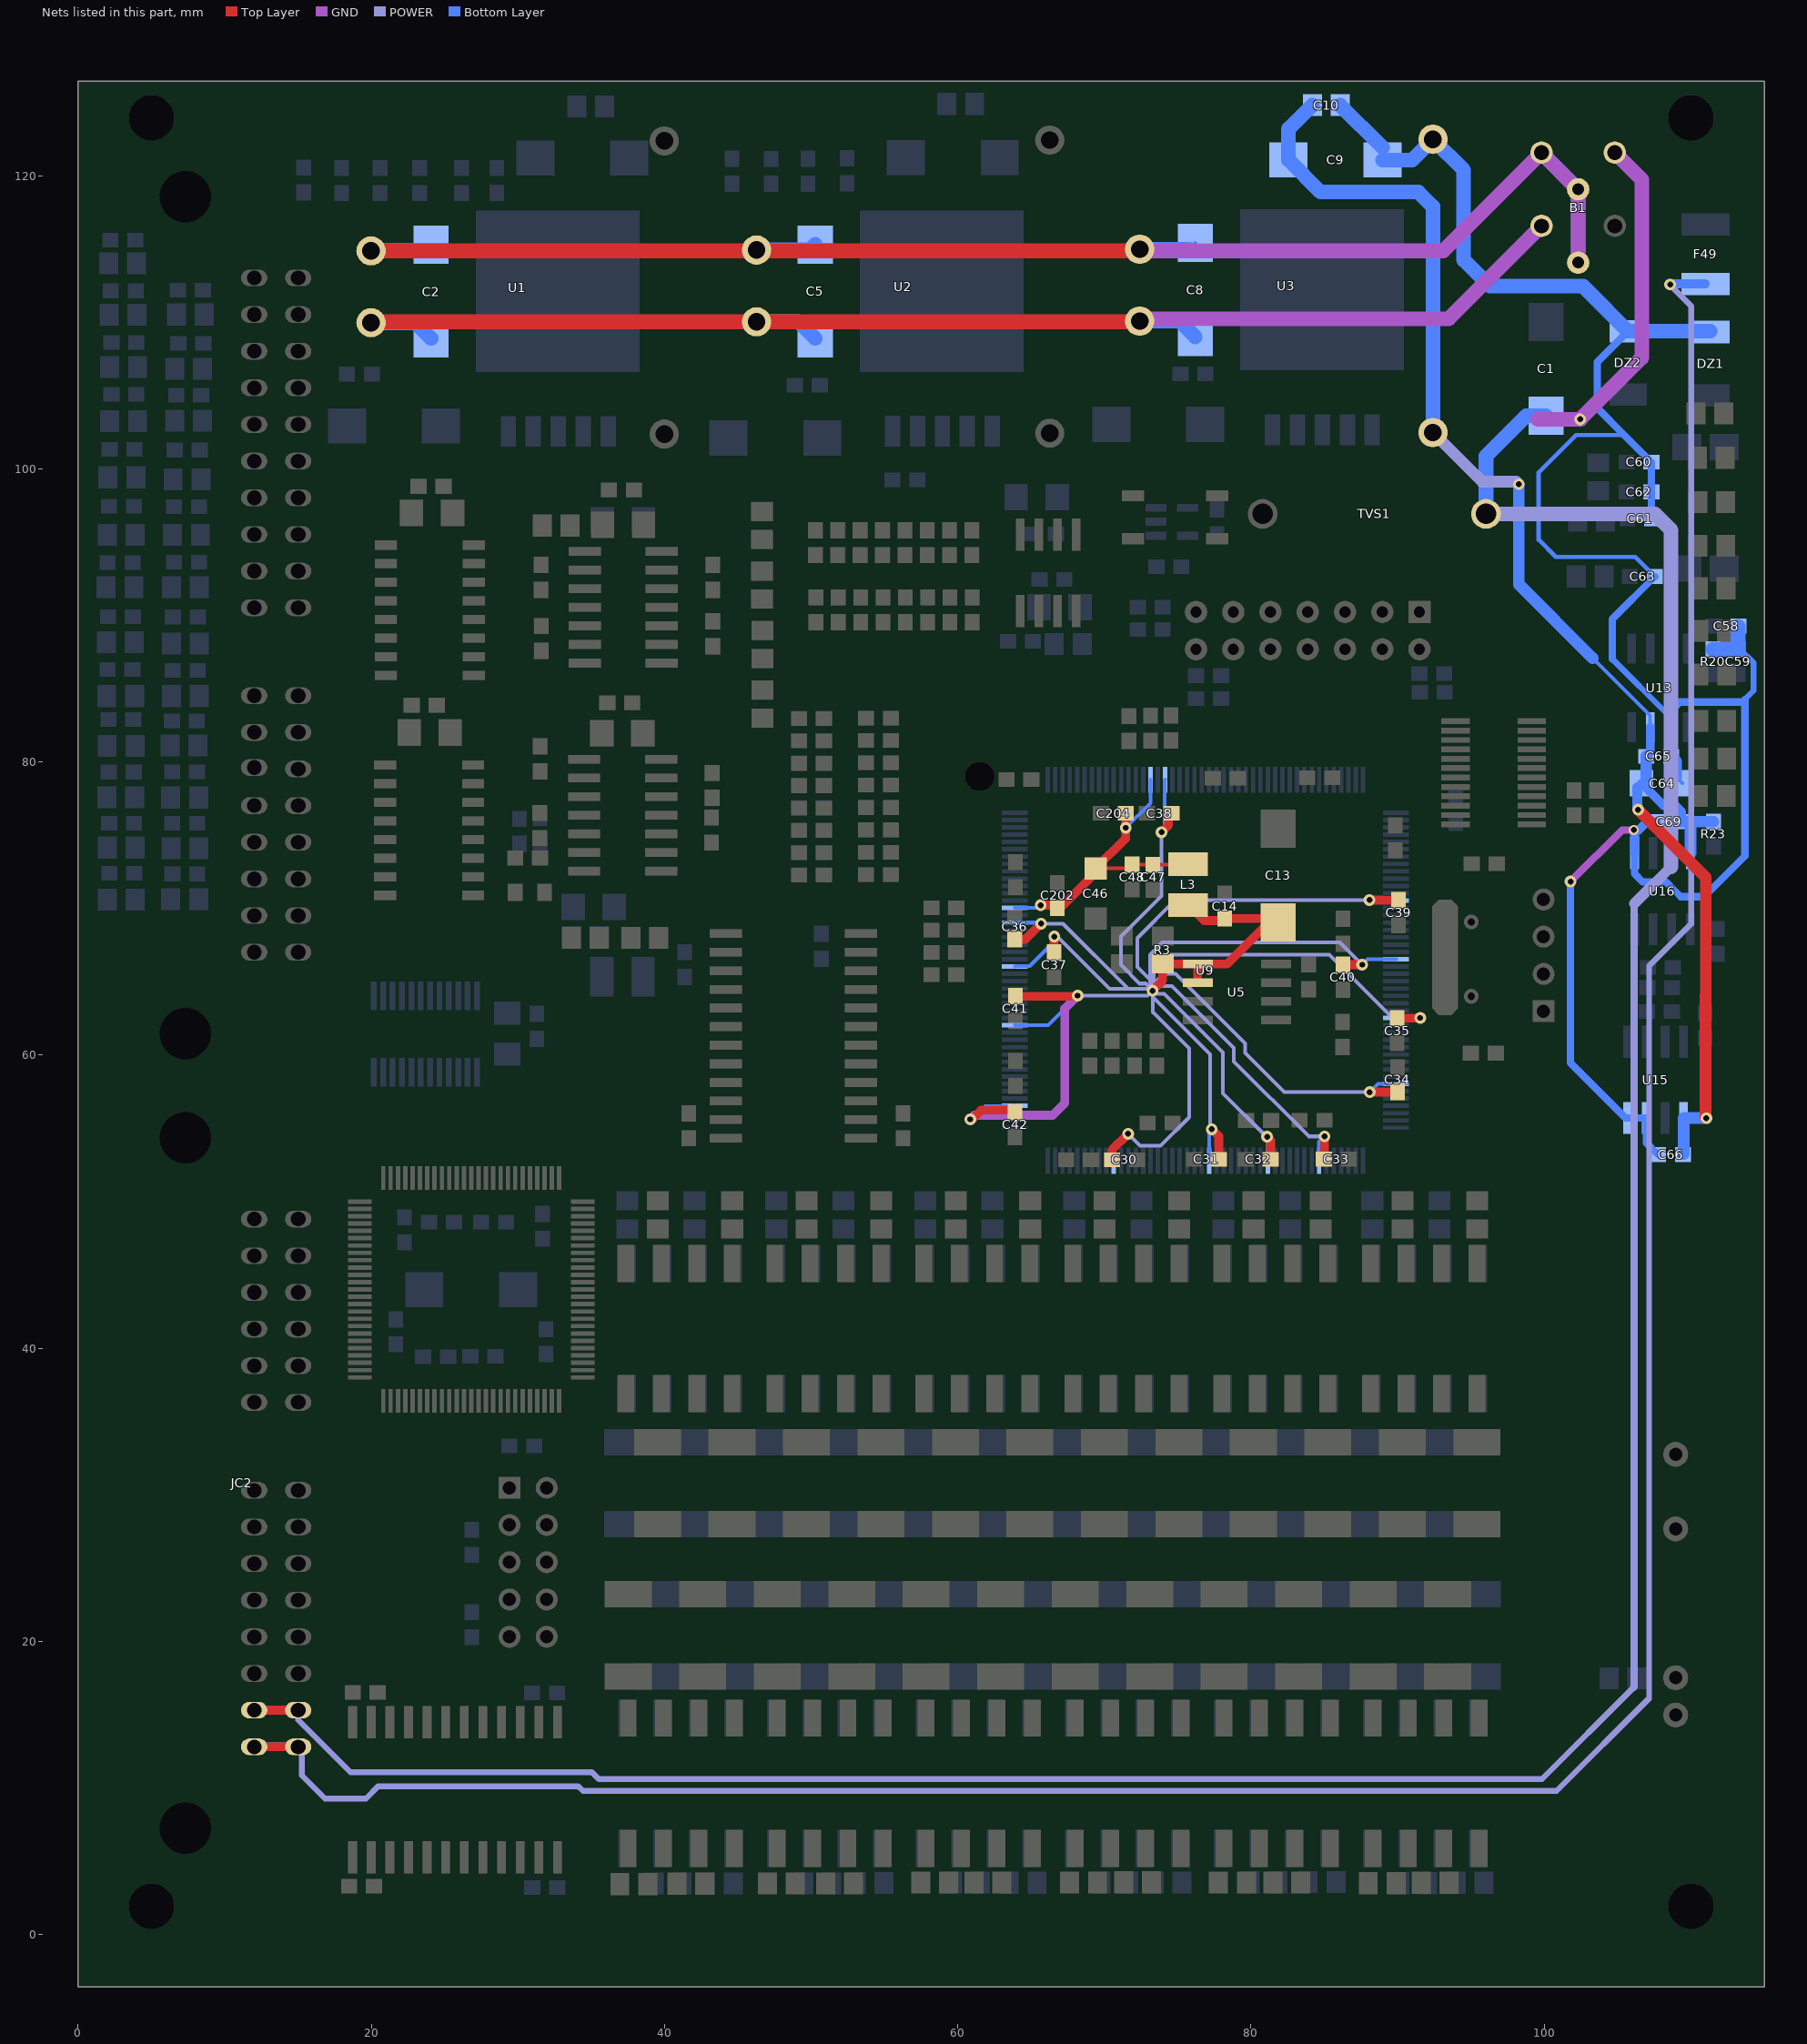
[diagram p0: the nets of this part, all layers, seen from the top]
# Altium PCB MISC86180.PCBDOC (part 3 of 9)
Units mm, origin at the board's own origin, x right, y up, seen from the top; angles counter-clockwise.
Board outline 115 x 130 mm, 4 copper layers (Top Layer, GND, POWER, Bottom Layer); 475 components, 355 nets, 1755 pads, 459 vias.

## Footprints (in the part's own frame and the unit in brackets; to place one, negate y for a bottom-side part, rotate by r counter-clockwise, add the part's x,y. Pads: shape width x height; smd on the part's side, far side on the other; paste and mask are expansions set on the pad) (continued)
AQZ102 [mm]
  round 1.7 hole 0.9: 1(1.275,-1.026) 2(3.815,-1.026) 3(13.975,-1.026) 4(19.055,-1.026)
  silkscreen extent 0,-3.06 20.32,-0.01
BNX012H [mm]
  round 1.524 hole 1: 1(-3,-3) 2(-3,-8) 3(-8,-3) 4(-8,-8)
  round 1.524 hole 0.8: 5(-5.5,-5.5) 6(-0.5,-5.5)
  silkscreen extent -12.19,-11.05 0,0
CR1608-0603 [mm]
  rect 1.1x1 smd: 1(-0.85,-0.018) 2(0.85,-0.018)
CR2012-0805 [mm]
  rect 1.3x1.5 smd: 1(-0.941,-0.018) 2(0.959,-0.018)
CR3216-1206 [mm]
  rect 1.6x1.8 smd: 1(-1.391,-0.018) 2(1.409,-0.018)
  silkscreen extent -0.29,-0.82 0.31,0.78
CR3225-1210 [mm]
  rect 1.6x2.7 smd: 1(-1.395,0.005) 2(1.405,0.005)
  silkscreen extent -0.3,-1.25 0.3,1.25
CR6332-2512 [mm] "Chip Resistor; Body 6.3 x 3.2 mm (LxW typ)"
  rect 1.8x3.2 smd: 1(-2.8,0) 2(2.8,0)
  silkscreen extent -1.6,-1.5 1.6,1.5
D008 [mm]
  rect 0.6x2.05 smd: 1(-1.9,-2.673) 2(-0.63,-2.673) 3(0.64,-2.673) 4(1.91,-2.673) 5(1.91,2.677) 6(0.64,2.677) 7(-0.63,2.677) 8(-1.9,2.677)
  silkscreen extent -2.88,-2.8 2.5,1.25
DBQ024 [mm]
  rect 0.4x1.95 smd: 1(-3.522,-2.616) 2(-2.882,-2.616) 3(-2.242,-2.616) 4(-1.602,-2.616) 5(-0.962,-2.616) 6(-0.322,-2.616) 7(0.318,-2.616) 8(0.958,-2.616) 9(1.598,-2.616) 10(2.238,-2.616) 11(2.878,-2.616) 12(3.518,-2.616) 13(3.518,2.584) 14(2.878,2.584) 15(2.238,2.584) 16(1.598,2.584) 17(0.958,2.584) 18(0.318,2.584) 19(-0.322,2.584) 20(-0.962,2.584) 21(-1.602,2.584) 22(-2.242,2.584) 23(-2.882,2.584) 24(-3.522,2.584)
  silkscreen extent -4.4,-2.74 4.37,1.21
DBV005 [mm]
  rect 0.55x1.45 smd: 1(-0.941,-1.094) 2(0.009,-1.094) 3(0.959,-1.094) 4(0.959,1.056) 5(-0.941,1.056)
  silkscreen extent -1.57,-1.37 1.56,0.88
DCDC_5W [mm]
  round 2 hole 1.2: 1(14.991,-15.832) 2(14.991,-10.932) 3(34.991,-23.432) 4(34.991,-3.432)
  silkscreen extent 12.05,-26.01 37.5,-0.01
FUSE [mil]
  rect 60x130 smd: 1(10.18,-65.41) 2(170.18,-65.41)
  silkscreen extent 0,-135 180,5
HDR1X4 [mm] "Connector; Header; 4 Position"
  rect 1.5x1.5 hole 0.9: 1(0,0)
  round 1.5 hole 0.9: 2(2.54,0) 3(5.08,0) 4(7.62,0)
  silkscreen extent -1.27,-1.27 8.89,1.27
HDR2X5 [mm]
  rect 1.5x1.5 hole 0.9: 1(0.005,0.005)
  round 1.5 hole 0.9: 2(0.005,2.545) 3(2.545,0.005) 4(2.545,2.545) 5(5.085,0.005) 6(5.085,2.545) 7(7.625,0.005) 8(7.625,2.545) 9(10.165,0.005) 10(10.165,2.545)
  silkscreen extent -1.27,-1.27 11.43,3.81
INDC2012-0805 [mm]
  rect 1x1.2 smd: 1(-0.995,-0.008) 2(1.005,-0.008)
  silkscreen extent -0.2,-0.51 0.2,0.49
JTAG14 [mil]
  rect 60x60 hole 30: 1(0,0)
  round 60 hole 30: 2(0,100) 3(100,0) 4(100,100) 5(200,0) 6(200,100) 7(300,0) 8(300,100) 9(400,0) 10(400,100) 11(500,0) 12(500,100) 13(600,0) 14(600,100)
  silkscreen extent -200,-125 800,225
Oscillator [mil]
  round 40 hole 20: 1(-200.19,-0.02) 2(-0.19,-0.02)
  oct 310x70 smd: 3(-105.19,-70.02)
  silkscreen extent -310,-85 110,85
QFP176NEW [mm]
  rect 0.3x1.778 smd: 1(-0.003,-0.011) 2(0.497,-0.011) 3(0.997,-0.011) 4(1.497,-0.011) 5(1.997,-0.011) 6(2.497,-0.011) 7(2.997,-0.011) 8(3.497,-0.011) 9(3.997,-0.011) 10(4.497,-0.011) 11(4.997,-0.011) 12(5.497,-0.011) 13(5.997,-0.011) 14(6.497,-0.011) 15(6.997,-0.011) 16(7.497,-0.011) 17(7.997,-0.011) 18(8.497,-0.011) 19(8.997,-0.011) 20(9.497,-0.011) 21(9.997,-0.011) 22(10.497,-0.011) 23(10.997,-0.011) 24(11.497,-0.011) 25(11.997,-0.011) 26(12.497,-0.011) 27(12.997,-0.011) 28(13.497,-0.011) 29(13.997,-0.011) 30(14.497,-0.011) 31(14.997,-0.011) 32(15.497,-0.011) 33(15.997,-0.011) 34(16.497,-0.011) 35(16.997,-0.011) 36(17.497,-0.011) 37(17.997,-0.011) 38(18.497,-0.011) 39(18.997,-0.011) 40(19.497,-0.011) 41(19.997,-0.011) 42(20.497,-0.011) 43(20.997,-0.011) 44(21.497,-0.011) 89(21.497,25.989) 90(20.997,25.989) 91(20.497,25.989) 92(19.997,25.989) 93(19.497,25.989) 94(18.997,25.989) 95(18.497,25.989) 96(17.997,25.989) 97(17.497,25.989) 98(16.997,25.989) 99(16.497,25.989) 100(15.997,25.989) 101(15.497,25.989) 102(14.997,25.989) 103(14.497,25.989) 104(13.997,25.989) 105(13.497,25.989) 106(12.997,25.989) 107(12.497,25.989) 108(11.997,25.989) 109(11.497,25.989) 110(10.997,25.989) 111(10.497,25.989) 112(9.997,25.989) 113(9.497,25.989) 114(8.997,25.989) 115(8.497,25.989) 116(7.997,25.989) 117(7.497,25.989) 118(6.997,25.989) 119(6.497,25.989) 120(5.997,25.989) 121(5.497,25.989) 122(4.997,25.989) 123(4.497,25.989) 124(3.997,25.989) 125(3.497,25.989) 126(2.997,25.989) 127(2.497,25.989) 128(1.997,25.989) 129(1.497,25.989) 130(0.997,25.989) 131(0.497,25.989) 132(-0.003,25.989)
  rect 1.778x0.3 smd: 45(23.747,2.239) 46(23.747,2.739) 47(23.747,3.239) 48(23.747,3.739) 49(23.747,4.239) 50(23.747,4.739) 51(23.747,5.239) 52(23.747,5.739) 53(23.747,6.239) 54(23.747,6.739) 55(23.747,7.239) 56(23.747,7.739) 57(23.747,8.239) 58(23.747,8.739) 59(23.747,9.239) 60(23.747,9.739) 61(23.747,10.239) 62(23.747,10.739) 63(23.747,11.239) 64(23.747,11.739) 65(23.747,12.239) 66(23.747,12.739) 67(23.747,13.239) 68(23.747,13.739) 69(23.747,14.239) 70(23.747,14.739) 71(23.747,15.239) 72(23.747,15.739) 73(23.747,16.239) 74(23.747,16.739) 75(23.747,17.239) 76(23.747,17.739) 77(23.747,18.239) 78(23.747,18.739) 79(23.747,19.239) 80(23.747,19.739) 81(23.747,20.239) 82(23.747,20.739) 83(23.747,21.239) 84(23.747,21.739) 85(23.747,22.239) 86(23.747,22.739) 87(23.747,23.239) 88(23.747,23.739) 133(-2.253,23.739) 134(-2.253,23.239) 135(-2.253,22.739) 136(-2.253,22.239) 137(-2.253,21.739) 138(-2.253,21.239) 139(-2.253,20.739) 140(-2.253,20.239) 141(-2.253,19.739) 142(-2.253,19.239) 143(-2.253,18.739) 144(-2.253,18.239) 145(-2.253,17.739) 146(-2.253,17.239) 147(-2.253,16.739) 148(-2.253,16.239) 149(-2.253,15.739) 150(-2.253,15.239) 151(-2.253,14.739) 152(-2.253,14.239) 153(-2.253,13.739) 154(-2.253,13.239) 155(-2.253,12.739) 156(-2.253,12.239) 157(-2.253,11.739) 158(-2.253,11.239) 159(-2.253,10.739) 160(-2.253,10.239) 161(-2.253,9.739) 162(-2.253,9.239) 163(-2.253,8.739) 164(-2.253,8.239) 165(-2.253,7.739) 166(-2.253,7.239) 167(-2.253,6.739) 168(-2.253,6.239) 169(-2.253,5.739) 170(-2.253,5.239) 171(-2.253,4.739) 172(-2.253,4.239) 173(-2.253,3.739) 174(-2.253,3.239) 175(-2.253,2.739) 176(-2.253,2.239)
  silkscreen extent -2.02,-0.51 22.35,24.88
SB560 [mil]
  round 80 hole 55: 1(0.18,-0.41) 2(600.18,-0.41)
  silkscreen extent 0,-100 600,100
SO16 [mm]
  rect 1.5x0.635 smd: 1(-0.007,-0.002) 2(-0.007,-1.272) 3(-0.007,-2.542) 4(-0.007,-3.812) 5(-0.007,-5.082) 6(-0.007,-6.352) 7(-0.007,-7.622) 8(-0.007,-8.892) 9(5.993,-8.892) 10(5.993,-7.622) 11(5.993,-6.352) 12(5.993,-5.082) 13(5.993,-3.812) 14(5.993,-2.542) 15(5.993,-1.272) 16(5.993,-0.002)
  silkscreen extent 0.99,-9.58 4.99,0.69
SO-G8 [mm]
  rect 0.6x2.2 smd: 1(-1.893,-2.599) 2(-0.623,-2.599) 3(0.647,-2.599) 4(1.917,-2.599) 5(1.917,2.601) 6(0.647,2.601) 7(-0.623,2.601) 8(-1.893,2.601)
  silkscreen extent -2.87,-2.72 2.51,1.1
SW_RESET [mil]
  rect 60x30 smd: 1(-25,-30) 2(-25,-145) 3(201,-145) 4(201,-30)
  silkscreen extent 0,-176 176,0
TC7343-2917 [mm]
  rect 2.6x2.4 smd: 1(-3.194,-0.018) 2(3.206,-0.018)
  silkscreen extent -4.57,-2.32 3.81,2.41
TQFP100 [mm]
  rect 1.6x0.3 smd: 1(-7.6,6) 2(-7.6,5.5) 3(-7.6,5) 4(-7.6,4.5) 5(-7.6,4) 6(-7.6,3.5) 7(-7.6,3) 8(-7.6,2.5) 9(-7.6,2) 10(-7.6,1.5) 11(-7.6,1) 12(-7.6,0.5) 13(-7.6,0) 14(-7.6,-0.5) 15(-7.6,-1) 16(-7.6,-1.5) 17(-7.6,-2) 18(-7.6,-2.5) 19(-7.6,-3) 20(-7.6,-3.5) 21(-7.6,-4) 22(-7.6,-4.5) 23(-7.6,-5) 24(-7.6,-5.5) 25(-7.6,-6) 51(7.6,-6) 52(7.6,-5.5) 53(7.6,-5) 54(7.6,-4.5) 55(7.6,-4) 56(7.6,-3.5) 57(7.6,-3) 58(7.6,-2.5) 59(7.6,-2) 60(7.6,-1.5) 61(7.6,-1) 62(7.6,-0.5) 63(7.6,0) 64(7.6,0.5) 65(7.6,1) 66(7.6,1.5) 67(7.6,2) 68(7.6,2.5) 69(7.6,3) 70(7.6,3.5) 71(7.6,4) 72(7.6,4.5) 73(7.6,5) 74(7.6,5.5) 75(7.6,6)
  rect 0.3x1.6 smd: 26(-6,-7.6) 27(-5.5,-7.6) 28(-5,-7.6) 29(-4.5,-7.6) 30(-4,-7.6) 31(-3.5,-7.6) 32(-3,-7.6) 33(-2.5,-7.6) 34(-2,-7.6) 35(-1.5,-7.6) 36(-1,-7.6) 37(-0.5,-7.6) 38(0,-7.6) 39(0.5,-7.6) 40(1,-7.6) 41(1.5,-7.6) 42(2,-7.6) 43(2.5,-7.6) 44(3,-7.6) 45(3.5,-7.6) 46(4,-7.6) 47(4.5,-7.6) 48(5,-7.6) 49(5.5,-7.6) 50(6,-7.6) 76(6,7.6) 77(5.5,7.6) 78(5,7.6) 79(4.5,7.6) 80(4,7.6) 81(3.5,7.6) 82(3,7.6) 83(2.5,7.6) 84(2,7.6) 85(1.5,7.6) 86(1,7.6) 87(0.5,7.6) 88(0,7.6) 89(-0.5,7.6) 90(-1,7.6) 91(-1.5,7.6) 92(-2,7.6) 93(-2.5,7.6) 94(-3,7.6) 95(-3.5,7.6) 96(-4,7.6) 97(-4.5,7.6) 98(-5,7.6) 99(-5.5,7.6) 100(-6,7.6)
  silkscreen extent -7.72,-6.4 6.4,6.82
WSO24 [mm] "Small Outline; 24 Leads; Body Width 7.5 mm; Pitch 1.27 mm"
  rect 0.6x2.2 smd: 1(-6.985,-4.6) 2(-5.715,-4.6) 3(-4.445,-4.6) 4(-3.175,-4.6) 5(-1.905,-4.6) 6(-0.635,-4.6) 7(0.635,-4.6) 8(1.905,-4.6) 9(3.175,-4.6) 10(4.445,-4.6) 11(5.715,-4.6) 12(6.985,-4.6) 13(6.985,4.6) 14(5.715,4.6) 15(4.445,4.6) 16(3.175,4.6) 17(1.905,4.6) 18(0.635,4.6) 19(-0.635,4.6) 20(-1.905,4.6) 21(-3.175,4.6) 22(-4.445,4.6) 23(-5.715,4.6) 24(-6.985,4.6)
  silkscreen extent -7.96,-4.73 7.93,3.1
ZJYS [mm]
  rect 1.8x2 smd: 1(0.009,-0.015) 2(0.009,-2.555) 3(8.309,-2.555) 4(8.309,-0.015)
  silkscreen extent 1.74,-3.83 6.57,1.25

## Part data
C1 C2 C3 C5 C6 C8 C9 C11 C13 C15 C17 C81: "Polarized Capacitor (Surface Mount)"
C4 C7 C10 C12 C14 C16 C18 C19 C20 C21 C22 C23 C24 C25 C26 C27 C28 C29 C30 C31 C32 C33 C34 C35 C36 C37 C38 C39 C40 C41 C42 C46 C47 C48 C52 C53 C54 C55 C56 C57 C58 C59 C60 C61 C62 C63 C64 C65 C66 C67 C68 C69 C82 C83 C84 C85 C86 C87 C88 C89 C90 C91 C92 C93 C94 C95 C96 C97 C98 C99 C100 C101 C102 C103 C104 C105 C106 C107 C108 C109 C110 C111 C112 C113 C114 C115 C116 C117 C118 C119 C120 C121 C122 C123 C124 C125 C126 C127 C128 C129 C130 C131 C132 C133 C134 C135 C136 C137 C138 C139 C140 C141 C142 C143 C144 C145 C146 C147 C148 C149 C150 C151 C152 C153 C154 C155 C156 C157 C158 C159 C160 C161 C162 C163 C164 C165 C166 C167 C168 C169 C170 C171 C172 C173 C174 C175 C176 C177 C178 C179 C180 C181 C182 C183 C184 C185 C186 C187 C188 C189 C191 C192 C195 C196 C197 C199 C200 C201 C202 C203 C204 C205 C206 C208 C209: "Capacitor"
D1 D2 D3 D4 D5 D6 D7 D8 D9 D10: library part LED1, "Typical YELLOW GaAs LED"
DZ1 DZ2: library part AK1B
F1 F2 F3 F4 F5 F6 F7 F8 F9 F10 F11 F12 F13 F14 F15 F16 F17 F18 F19 F20 F21 F22 F23 F24 F25 F26 F27 F28 F29 F30 F31 F32 F33 F34 F35 F36 F37 F38 F39 F40 F41 F42 F43 F44 F45 F46 F47 F48 R1 R2 R3 R4 R5 R6 R7 R8 R9 R10 R11 R12 R13 R14 R17 R18 R19 R20 R21 R22 R23 R24 R33 R34 R35 R36 R37 R38 R41 R42 R43 R44 R45 R46 R47 R48 R49 R50 R51 R52 R53 R54 R55 R56 R57 R58 R59 R60 R61 R62 R63 R64 R65 R66 R67 R68 R69 R70 R71 R72 R73 R74 R75 R76 R77 R78 R79 R80 R81 R82 R83 R84 R85 R86 R87 R88 R89 R90 R91 R92 R93 R94 R95 R96 R97 R98 R99 R100 R101 R102 R103 R104 R105 R106 R107 R108 R109 R110 R111 R112 R113 R114 R115 R116 R117 R118 R119 R120 R121 R122 R123 R124 R125 R126 R127 R128 R129 R130 R131 R132 R133 R134 R136 R137 R138 R139 R140 R141 R142 R143 R144 R145 R146 R147 R148 R149 R150 R151 R152 R153 R154 R155 R156 R157 R158 R159 R160 R161 R162 R163 R164 R165 R166 R167 R168 R170 R171 R172 R173 R180 R181: "Resistor"
F49: library part FUSE1, "Fuse"
J1: library part "Header 7X2A", "Header, 7-Pin, Dual row"
J2: "Header, 4-Pin"
J3: library part "Header 5X2", "Header, 5-Pin, Dual row"
JC1: library part CJ20
JC2: library part CJ10
SW1: "Switch"
TVS1: library part diode2
U1 U2 U3: library part DCDC
U10 U20: "10-Bit FET Bus Switch with Level Shifting"
U19: "MAX II 2.5/3.3V CPLD, 80 I/Os, 100-Pin Plastic TQFP, Pb-Free, Commercial Temperature, Speed Grade 5"
U21 U22 U23 U24: "Octal Bus Transceiver and 3.3-V to 5-V Shifter with 3-State Outputs"
U25 U26 U27 U28: library part M74HC4053M1R, "Analog Multiplexer/Demultiplexer Triple 2-Channel"
U29 U30 U31 U32: library part LM324D, "Quad Low-Power Operational Amplifier"
U34: library part ADR421
U35: library part AQZ
Y1: library part CRYSTAL, "Crystal"

## Free pads (board coordinates)
  round 3.1 hole 3.1: 1(5.01,123.95) 2(5.01,1.95) 3(110.01,1.95) 4(110.01,123.95)
  round 2 hole 2: 5(61.49,79.01)

## Via types
v1: diameter 0.8, hole 0.4, Top Layer to Bottom Layer, 339 vias
v2: diameter 0.7, hole 0.4, Top Layer to Bottom Layer, 83 vias
v3: diameter 0.5, hole 0.254, Top Layer to Bottom Layer, 37 vias

## Nets (pads, with @x,y where several pads share a name; then routed paths per layer and width w, separated by ;. In a path a pad name is that pad's centre, name@x,y a point inside that pad or via, vN(x,y) a via of type N, cw(c..) or ccw(c..) an arc to the next point about the centre after c; other vN are vias at no path point)
5VO1+: C9.1 C10.2 C64.2 C65.2 C66.2 C69.2 R23.2 U3.3 U13.3 U15.1 U16.8 | length 101
  Top Layer w0.8: v1(106.4,76.74) 111.01,72.13 111.01,64.134 111,64.124 111,55.75 v1(111.05,55.7)
  POWER w0.254: v1@98.089,98.95 v1(98.26,98.95)
  POWER w0.8: U3.3@92.405,102.478 95.761,99.121 v1@98.089,99.121
  Bottom Layer w0.254: C9.1@82.556,120.684 C9.1@82.556,121.068 ; v1@98.24,98.93 v1(98.26,98.95) ; 103.295,87.085 107.22,83.16 U13.3@107.22,82.377 ; v1@106.34,76.8 v1(106.4,76.74) ; C64.2@106.34,78.261 C64.2@106.621,78.542 C64.2@106.95,78.871 ; C69.2@109.234,75.928 C69.2@109.36,75.928 C69.2@109.68,75.608 ; v1@111.037,55.713 v1(111.05,55.7)
  Bottom Layer w0.6: C64.2@106.621,78.542 108.134,77.028 108.952,77.028 109.36,76.62 C69.2@109.36,75.928 ; C65.2@106.95,80.382 107.22,80.652 U13.3@107.22,82.377
  Bottom Layer w0.7: v1@106.34,76.8 C64.2@106.34,78.261
  Bottom Layer w0.8: v1(98.26,98.95) 98.26,92.12 103.295,87.085 ; C64.2@106.95,78.871 C65.2@106.95,80.382 ; C69.2@109.36,75.928 R23.2@111.54,75.928 ; C66.2@109.501,53.26 U15.1@109.501,55.713 v1@111.037,55.713 ; U16.8@109.963,73.791 109.963,75.892
  Bottom Layer w1: C10.2@84.181,124.812 82.556,123.187 C9.1@82.556,121.068 84.744,118.88 91.41,118.88 92.405,117.885 U3.3@92.405,102.478
5VO1-: C9.2 C10.1 C58.1 C59.1 C60.1 C61.1 C62.1 C63.1 C64.1 C65.1 C66.1 C69.1 DZ1.2 DZ2.2 R20.1 U3.4 U13.2 U15.3 U15.4 U16.5 | length 156.1
  GND w0.5: v1(101.79,71.84) 105.31,75.36 v2(106.1,75.36)
  Bottom Layer w0.254: C9.2@88.956,121.068 C9.2@88.956,121.937 ; 102.64,112.18 102.93,112.18 ; 105.18,102.3 105.45,102.3 ; U16.5@106.15,73.787 U16.5@106.153,73.791 ; v2@106.153,75.253 v2@106.26,75.36 ; C61.1@107.31,96.642 C61.1@107.37,96.582 ; C65.1@108.49,80.542 C65.1@108.65,80.382 ; C64.1@108.981,78.981 C64.1@109.421,78.542 ; DZ1.2@111.3,109.39 DZ1.2@111.36,109.33 ; R20.1@111.49,87.672 R20.1@111.508,87.69 ; C59.1@113.218,87.69 C59.1@113.25,87.722 ; C58.1@113.25,89.24 C58.1@113.25,89.272
  Bottom Layer w0.3: 105.18,102.3 102.16,102.3 99.62,99.76 99.62,95.16 100.79,93.99 106.2,93.99 C63.1@107.54,92.65
  Bottom Layer w0.4: 104.64,87.02 U13.2@108.41,83.25 ; C59.1@113.346,87.69 114.268,86.768 114.268,84.858 113.68,84.27
  Bottom Layer w0.5: v1(101.79,71.84) 101.79,59.46 105.537,55.713 U15.3@106.961,55.713 106.961,54.017 C66.1@107.76,53.218 ; 104.64,87.02 104.64,89.75 C63.1@107.54,92.65 ; DZ2.2@105.72,109.39 103.61,107.28 103.61,104.14 105.45,102.3 107.31,100.44 C62.1@107.31,98.422 C61.1@107.31,96.642 ; U16.5@106.15,73.787 106.15,72.37 106.7,71.82 108.29,71.82 108.84,71.27 108.843,71.27 109.303,70.81 110.9,70.81 113.68,73.59 113.68,84.27 ; U13.2@108.41,83.25 109.25,84.09 113.62,84.09 ; U13.2@108.49,82.377 U13.2@108.49,83.33 ; C59.1@113.218,87.59 C59.1@113.218,87.69 C59.1@113.346,87.69
  Bottom Layer w0.6: v2(106.1,75.36) 106.26,75.36 106.434,75.36 107.002,75.928 C69.1@107.66,75.928 ; U16.5@106.153,73.791 106.153,75.253 v2@106.153,75.307 ; C65.1@108.49,80.542 U13.2@108.49,82.377
  Bottom Layer w0.8: C65.1@108.65,80.382 108.981,80.05 C64.1@108.981,78.981
  Bottom Layer w1: C10.1@86.081,124.812 C9.2@88.956,121.937 ; C9.2@88.956,121.068 90.995,121.068 U3.4@92.405,122.478 92.405,122.475 94.5,120.38 94.5,114.25 96.28,112.47 102.64,112.47 102.93,112.18 DZ2.2@105.72,109.39 DZ1.2@111.3,109.39 ; R20.1@111.508,87.69 C59.1@113.218,87.69 C58.1@113.218,89.24
12V+: B1.2 C2.1 C5.1 C8.1 U1.1 U2.1 U3.1 | length 95.8
  Top Layer w1: U1.1@19.981,109.968 20.041,110.028 U2.1@46.271,110.028 72.355,110.028 U3.1@72.405,110.078 U3.1@72.567,110.24
  GND w1: U3.1@72.567,110.24 93.48,110.24 B1.2@99.81,116.57
  Bottom Layer w1: U1.1@19.981,109.968 22.994,109.968 C2.1@24.072,108.89 ; U2.1@46.271,110.028 49.144,110.028 C5.1@50.272,108.9 ; U3.1@72.405,110.078 75.114,110.078 C8.1@76.192,109
12V-: B1.4 B1.5 B1.6 C2.2 C5.2 C8.2 U1.2 U2.2 U3.2 | length 137.8
  Top Layer w0.254: U2.2@46.211,114.868 U2.2@46.271,114.928 U3.2@72.355,114.928 ; U3.2@72.405,114.978 U3.2@72.477,115.05
  Top Layer w1: U1.2@19.981,114.868 U3.2@72.405,114.868 ; B1.4@99.81,121.54 B1.4@99.81,121.57 ; B1.5@102.28,119.07 B1.5@102.31,119.07
  GND w1: U3.2@72.405,114.868 93.108,114.868 B1.4@99.81,121.57 ; B1.4@99.81,121.54 B1.5@102.28,119.07 ; B1.6@102.31,114.07 B1.5@102.31,119.07
  Bottom Layer w0.254: C8.2@75.769,114.978 C8.2@76.192,115.4
  Bottom Layer w1: U1.2@19.981,114.868 C2.2@23.649,114.868 ; U2.2@46.271,114.928 49.899,114.928 C5.2@50.272,115.3 ; U3.2@72.405,114.978 C8.2@75.769,114.978 ; B1.4@99.81,121.57 B1.5@102.31,119.07 B1.6@102.31,114.07
12VIN+: F49.2 JC2.26 JC2.34 | length 204.5
  Top Layer w0.6: JC2.34@12.01,12.814 JC2.26@15.01,12.814
  POWER w0.254: v1@108.58,112.5 v1@108.62,112.5
  POWER w0.4: JC2.26@15.01,12.814 15.27,12.554 15.27,10.86 16.84,9.29 19.64,9.29 20.48,10.13 34.1,10.13 34.43,9.8 100.83,9.8 107.15,16.12 107.15,66.09 110.02,68.96 110.02,111.1 v1@108.62,112.5
  Bottom Layer w0.254: v1@108.47,112.5 v1@108.47,112.54 ; F49.2@110.989,112.62 F49.2@110.991,112.617
  Bottom Layer w0.4: v1@108.47,112.5 v1@108.587,112.617
  Bottom Layer w0.6: JC2.34@12.01,12.814 JC2.26@15.01,12.814 ; v1@108.587,112.617 F49.2@110.991,112.617
  other v1: 108.58,112.57
12VIN-: B1.3 C1.2 JC2.25 JC2.33 TVS1.1 | length 230
  Top Layer w0.6: JC2.33@12.01,15.314 JC2.25@15.01,15.314
  GND w1: 99.55,103.38 v1(102.45,103.38) 106.65,107.58 106.65,119.73 B1.3@104.81,121.57
  POWER w0.254: 108.65,72.85 108.65,72.86
  POWER w0.4: JC2.25@15.01,15.314 15.01,14.658 18.588,11.08 35.04,11.08 35.51,10.61 99.84,10.61 106.1,16.87 ; 106.14,16.91 106.14,17.01
  POWER w0.5: 106.1,16.87 106.14,16.91 ; 106.14,17.01 106.14,70.33
  POWER w0.7: 106.14,70.33 106.14,70.34 108.65,72.85
  POWER w1: TVS1.1@96.025,96.92 107.55,96.92 108.65,95.82 108.65,72.86
  Bottom Layer w0.254: C1.2@100.428,103.314 C1.2@100.488,103.374
  Bottom Layer w0.6: JC2.33@12.01,15.314 JC2.25@15.01,15.314
  Bottom Layer w1: TVS1.1@96.025,96.92 96.025,100.865 98.784,103.624 C1.2@100.118,103.624 ; C1.2@100.362,103.38 v1(102.45,103.38)
+1.9VA: C46.2 C47.2 C48.2 C202.2 C204.2 L3.2 U9.31 U9.59 | length 22
  Top Layer w0.254: C202.2@66.602,70.23 C202.2@66.792,70.04 ; C46.2@69.4,72.648 C46.2@69.4,72.736 ; C46.2@69.4,72.79 C46.2@69.4,72.736 ; L3.2@75.671,73 C48.2@71.888,73 71.624,72.736 C46.2@69.4,72.736
  Top Layer w0.6: v1(65.65,70.23) C202.2@66.602,70.23 ; C202.2@66.792,70.04 66.99,70.04 69.4,72.449 C46.2@69.4,72.648 ; C46.2@69.4,72.736 71.46,74.796 C204.2@71.46,76.492
  Bottom Layer w0.254: U9.31@63.889,70.043 65.463,70.043 v1(65.65,70.23) ; v1(71.45,75.51) 73.139,77.199 U9.59@73.139,78.793
+1.9VD: C13.1 C14.2 C30.2 C31.2 C32.2 C33.2 C34.2 C35.2 C36.2 C37.2 C38.2 C39.2 C40.2 C41.2 C42.2 L3.1 R3.2 U5.5 U5.6 U9.4 U9.15 U9.23 U9.29 U9.61 U9.101 U9.109 U9.117 U9.126 U9.139 U9.146 U9.154 U9.167 | length 264.5
  Top Layer w0.254: v1@68.134,64.024 v1(68.17,64.06) ; v1(73.89,75.21) v1@73.985,75.305 ; U5.6@76.363,64.94 76.363,65.31 ; v1(77.32,54.95) v1@77.445,54.825 ; C13.1@81.538,69.056 C13.1@81.693,69.211 ; C33.2@84.96,52.908 C33.2@84.96,52.958 ; v1(88.09,57.48) v1@88.24,57.48 ; C39.2@90.048,70.57 C39.2@90.058,70.57
  Top Layer w0.6: v1(60.85,55.62) 60.97,55.62 61.6,56.25 63.768,56.25 C42.2@63.908,56.11 ; C36.2@63.882,67.912 64.622,67.912 v1(65.68,68.97) ; C41.2@63.918,64.024 v1@68.134,64.024 ; C37.2@66.568,67.01 v1@66.568,68.078 ; C30.2@70.52,52.868 70.52,53.53 v1(71.62,54.63) ; v1(73.28,64.4) 73.972,65.092 R3.2@73.972,66.231 73.993,66.21 U5.5@76.363,66.21 ; v1@73.985,75.305 74.36,75.68 C38.2@74.36,76.472 ; L3.1@75.705,70.235 75.755,70.235 76.81,69.18 78.072,69.18 C14.2@78.212,69.32 C13.1@81.584,69.32 ; 76.363,65.31 U5.5@76.363,66.21 ; v1@77.445,54.825 77.8,54.47 C31.2@77.8,52.902 ; v1(81.09,54.43) 81.34,54.18 C32.2@81.34,52.902 ; C13.1@81.693,69.211 C13.1@81.848,69.056 81.538,69.056 81.206,69.056 78.36,66.21 U5.5@76.363,66.21 ; C33.2@85.01,52.958 v1(85.01,54.46) ; C40.2@86.258,66.17 v1(87.58,66.17) ; v1(88.07,70.58) C39.2@90.048,70.58 ; v1@88.24,57.48 C34.2@89.982,57.48 ; C35.2@89.968,62.52 v1@91.52,62.52
  GND w0.6: v1(60.85,55.62) 61.13,55.9 66.474,55.9 67.3,56.726 67.3,63.09 67.28,63.11 67.28,63.17 v1(68.17,64.06)
  POWER w0.254: v1(65.68,68.97) 67.17,68.97 71.62,64.52 ; v1(66.58,68.09) 66.78,68.09 70.35,64.52 71.62,64.52 ; v1(68.17,64.06) 72.94,64.06 v1(73.28,64.4) ; v1(71.62,54.63) 72.44,53.81 73.82,53.81 75.77,55.76 75.77,60.46 73.3,62.93 73.3,63.97 ; 72.76,64.52 71.62,64.52 ; v1@73.28,64.475 v1@73.28,64.42 ; v1(73.89,75.21) 73.89,70.86 71.13,68.1 71.13,66.16 72.41,64.88 72.82,64.88 v1@73.18,64.52 ; v1(77.32,54.95) 77.2,55.07 77.2,60.07 73.3,63.97 ; v1(81.09,54.43) 81.04,54.43 78.08,57.39 78.08,60.17 74.07,64.18 73.52,64.18 v1@73.29,64.41 ; v1(85.01,54.46) 83.93,54.46 78.82,59.57 78.82,60.49 74.6,64.71 73.59,64.71 v1@73.355,64.475 ; v1(87.58,66.17) 86.06,67.69 73.96,67.69 73.11,66.84 73.11,65.15 ; v1(88.07,70.58) 74.83,70.58 72.235,67.985 72.235,66.025 73.11,65.15 ; v1(88.09,57.48) 82.26,57.48 79.59,60.15 79.59,60.81 74.84,65.56 74.05,65.56 73.355,64.865 ; v1(91.54,62.54) 89.66,62.54 85.34,66.86 74.53,66.86 73.355,65.685 73.355,64.865 ; 71.62,64.52 v1@73.18,64.52 ; 73.11,65.15 73.11,64.72 v1@73.18,64.65 ; 73.11,65.15 73.18,65.08 v1@73.18,64.65 ; v1@73.18,64.52 v1@73.18,64.65 ; v1@73.18,64.52 v1@73.28,64.42 ; v1@73.18,64.65 v1@73.355,64.475 ; v1(73.28,64.4) v1@73.29,64.41 ; v1(73.28,64.4) v1@73.3,64.4 ; v1(73.28,64.4) v1@73.28,64.42 ; v1@73.28,64.42 v1@73.29,64.41 ; v1@73.29,64.41 v1@73.3,64.4 ; 73.3,63.97 v1@73.3,64.4 ; v1@73.355,64.475 73.355,64.865
  Bottom Layer w0.254: v1(60.85,55.62) 60.97,55.62 61.88,56.53 63.876,56.53 U9.4@63.889,56.543 ; U9.15@63.889,62.043 66.153,62.043 v1(68.17,64.06) ; U9.23@63.889,66.043 63.934,66.089 64.904,66.089 66.58,67.764 v1(66.58,68.09) ; U9.29@63.889,69.043 65.607,69.043 v1(65.68,68.97) ; U9.167@70.639,52.793 70.684,52.839 70.684,53.809 71.506,54.63 v1(71.62,54.63) ; v1(73.89,75.21) 74.11,75.43 74.11,78.764 U9.61@74.139,78.793 ; U9.154@77.139,52.793 v1@77.139,54.769 ; v1(81.09,54.43) 81.139,54.381 U9.146@81.139,52.793 ; U9.139@84.639,52.793 84.639,54.089 v1(85.01,54.46) ; v1(87.58,66.17) 87.953,66.543 U9.109@89.889,66.543 ; v1(88.09,57.48) 88.653,58.043 U9.126@89.889,58.043 ; v1@88.107,70.543 U9.101@89.889,70.543 ; U9.117@89.889,62.543 91.537,62.543 v1(91.54,62.54)